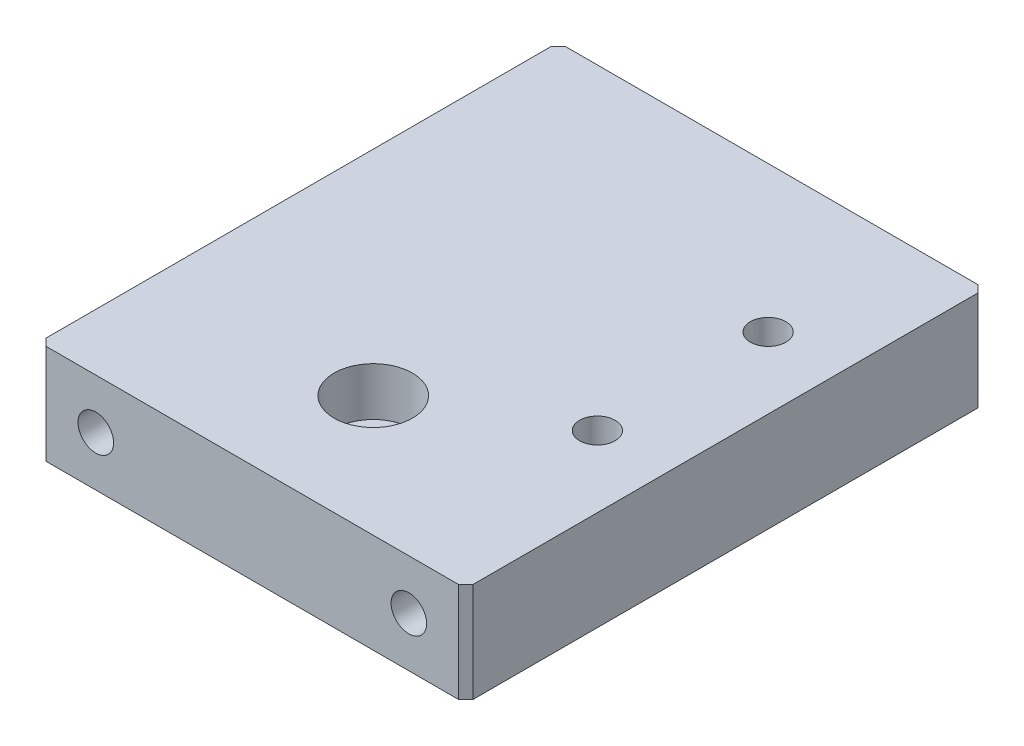
from build123d import *

# Parameters (mm, degrees)
SKETCH1_W                                            = 60
SKETCH1_H                                            = 73
BOSS_EXTRUDE1_DEPTH                                  = 7
M6_TAPPED_HOLE1_D                                    = 5
M6_TAPPED_HOLE1_DEPTH                                = 15
M6_TAPPED_HOLE1_TIP                                  = 1.502151548
M6_TAPPED_HOLE2_D                                    = 5
CHAMFER1_SIZE                                        = 1
HOLE_SIZE_PER_SOCKET_HEAD_CAP_SCREW_TYPE_D           = 6.6
HOLE_SIZE_PER_SOCKET_HEAD_CAP_SCREW_TYPE_CBORE_D     = 11
HOLE_SIZE_PER_SOCKET_HEAD_CAP_SCREW_TYPE_CBORE_DEPTH = 6.8


with BuildPart() as part:
    # Sketch1 → Boss-Extrude1 (new, symmetric)
    with BuildSketch(Plane(origin=(0, 0, 0), x_dir=(1, 0, 0), z_dir=(0, 1, 0))):
        Rectangle(SKETCH1_W, SKETCH1_H)
    extrude(amount=BOSS_EXTRUDE1_DEPTH, both=True)

    # M6 Tapped Hole1
    with Locations(Plane.XY.offset(36.5)):
        with Locations((22, 0), (-22, 0)):
            Hole(M6_TAPPED_HOLE1_D / 2, depth=M6_TAPPED_HOLE1_DEPTH)
            with Locations((0, 0, -(M6_TAPPED_HOLE1_DEPTH + M6_TAPPED_HOLE1_TIP / 2))):  # 118° drill point
                Cone(0, M6_TAPPED_HOLE1_D / 2, M6_TAPPED_HOLE1_TIP, mode=Mode.SUBTRACT)

    # M6 Tapped Hole2 (through all)
    with Locations(Plane(origin=(0, 7, 0), x_dir=(1, 0, 0), z_dir=(0, 1, 0))):
        with Locations((20, -8), (20, 16)):
            Hole(M6_TAPPED_HOLE2_D / 2)

    # Chamfer1
    chamfer1_edges = [part.edges().sort_by_distance(p)[0] for p in [
        (30, 0, 36.5),
        (-30, 0, 36.5),
        (-30, 0, -36.5),
        (30, 0, -36.5),
    ]]
    chamfer(chamfer1_edges, length=CHAMFER1_SIZE)

    # Hole Size per Socket Head Cap Screw Type1 (through all)
    with Locations(Plane(origin=(0, 7, 0), x_dir=(1, 0, 0), z_dir=(0, 1, 0))):
        with Locations((0, -19.5)):
            CounterBoreHole(HOLE_SIZE_PER_SOCKET_HEAD_CAP_SCREW_TYPE_D / 2, HOLE_SIZE_PER_SOCKET_HEAD_CAP_SCREW_TYPE_CBORE_D / 2, HOLE_SIZE_PER_SOCKET_HEAD_CAP_SCREW_TYPE_CBORE_DEPTH)


solid = part.part
